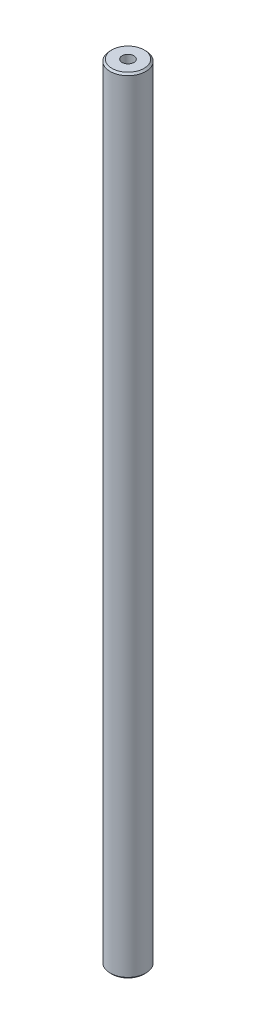
SolidWorks part; units mm, degrees
ref_plane "Front Plane" through (0, 0, 0) normal (0, 0, 1) x (1, 0, 0)
ref_plane "Top Plane" through (0, 0, 0) normal (0, 1, 0) x (1, 0, 0)
ref_plane "Right Plane" through (0, 0, 0) normal (1, 0, 0) x (0, 0, -1)
sketch "Sketch1" plane through (0, 0, 0) normal (0, 1, 0) x (1, 0, 0)
  circle A0 centre (0, 0) radius 5
  dimension "D1" = 10
extrude "Boss-Extrude1" add sketch "Sketch1" along normal mid plane 220
chamfer "Chamfer1" distance 0.5 angle 45 2 edges at (0, -110, 5) (0, 110, 5)
hole_wizard "M4 Tapped Hole1" positions "Sketch2" profile "Sketch3" tap size "M4" standard "GB"
sketch "Sketch2" plane through (0, 110, 0) normal (0, 1, 0) x (1, 0, 0)
  point P0 (0, 0)
sketch "Sketch3" plane through (0, 110, 0) normal (1, 0, 0) x (0, 0, 1)
  line L0 (0, 0) -> (0, 11.0914)
  line L1 (0, 11.0914) -> (1.65, 10.1)
  line L2 (1.65, 10.1) -> (1.65, 0)
  line L5 (1.65, 0) -> (0, 0)
  line L10 (0, 11.0914) -> (-1.65, 10.1) construction
  line L11 (0, -6.35) -> (0, 107.95) construction
  dimension "螺纹孔钻头直径" = 3.3
  dimension "螺纹孔钻头深度" = 10.1
  dimension "导头角度" = 118
cosmetic thread "Cosmetic Thread1" parameters "D1"=8, "D2"=4
hole_wizard "M4 Tapped Hole2" positions "Sketch4" profile "Sketch5" tap size "M4" standard "GB"
sketch "Sketch4" plane through (0, -110, 0) normal (0, -1, 0) x (-1, 0, 0)
  point P0 (0, 0)
sketch "Sketch5" plane through (0, -110, 0) normal (1, 0, 0) x (0, 0, -1)
  line L0 (0, 0) -> (0, 11.0914)
  line L1 (0, 11.0914) -> (1.65, 10.1)
  line L2 (1.65, 10.1) -> (1.65, 0)
  line L5 (1.65, 0) -> (0, 0)
  line L10 (0, 11.0914) -> (-1.65, 10.1) construction
  line L11 (0, -6.35) -> (0, 107.95) construction
  dimension "螺纹孔钻头直径" = 3.3
  dimension "螺纹孔钻头深度" = 10.1
  dimension "导头角度" = 118
cosmetic thread "Cosmetic Thread2"
